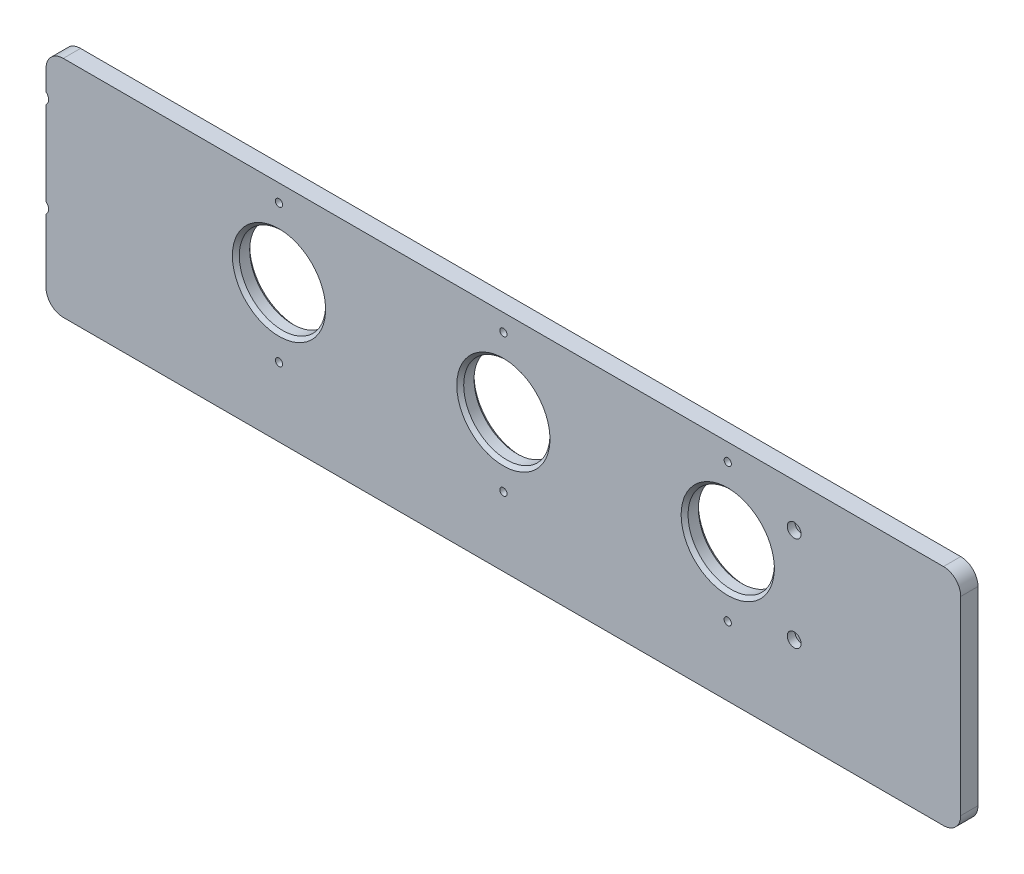
from build123d import *

# Parameters (mm, degrees)
SKETCH_1_W                   = 530
SKETCH_1_H                   = 130
EXTRUDE_1_DEPTH              = 10
HOLE_WIZARD_M4_1_D           = 4.5
HOLE_WIZARD_M4_1_CBORE_D     = 8
HOLE_WIZARD_M4_1_CBORE_DEPTH = 4.4
PATTERN_LINEAR_1_COUNT       = 2
PATTERN_LINEAR_1_PITCH       = 436
SKETCH_14_R                  = 25
CUT_EXTRUDE_1_DEPTH          = 274.03845883
CHAMFER_1_SIZE               = 2
HOLE_WIZARD_M5_2_D           = 4.2
FILLET_1_R                   = 10


with BuildPart() as part:
    # 草图1 → 凸台-拉伸1 (new body)
    with BuildSketch(Plane.XY):
        Rectangle(SKETCH_1_W, SKETCH_1_H)
    extrude(amount=EXTRUDE_1_DEPTH)

    # M4 六角凹头螺钉的柱形沉头孔1 (through all)
    with Locations(Plane(origin=(0, 0, 10), x_dir=(-1, 0, 0), z_dir=(0, 0, 1))):
        with Locations((-168.5, 15), (-168.5, -40)):
            hole_wizard_m4_1 = CounterBoreHole(HOLE_WIZARD_M4_1_D / 2, HOLE_WIZARD_M4_1_CBORE_D / 2, HOLE_WIZARD_M4_1_CBORE_DEPTH)

    # 阵列(线性)1: M4 六角凹头螺钉的柱形沉头孔1 ×2
    with Locations(*[(-i * PATTERN_LINEAR_1_PITCH, 0, 0) for i in range(1, PATTERN_LINEAR_1_COUNT)]):
        add(hole_wizard_m4_1, mode=Mode.SUBTRACT)

    # 草图14 → 切除-拉伸1 (cut, through all)
    with BuildSketch(Plane.XY.offset(10)):
        with Locations((-130, 15)):
            Circle(SKETCH_14_R)
        with Locations((0, 15)):
            Circle(SKETCH_14_R)
        with Locations((130, 15)):
            Circle(SKETCH_14_R)
    extrude(amount=-CUT_EXTRUDE_1_DEPTH, mode=Mode.SUBTRACT)

    # 倒角1
    chamfer_1_edges = [part.edges().sort_by_distance(p)[0] for p in [
        (-155, 15, 0),
        (-155, 15, 10),
        (-25, 15, 0),
        (-25, 15, 10),
        (105, 15, 0),
        (105, 15, 10),
    ]]
    chamfer(chamfer_1_edges, length=CHAMFER_1_SIZE)

    # M5 螺纹孔2 (through all)
    with Locations(Plane.XY.offset(10)):
        with Locations((130, 55), (-130, -25), (-130, 55), (0, 55), (0, -25), (130, -25)):
            Hole(HOLE_WIZARD_M5_2_D / 2)

    # 圆角1
    fillet_1_edges = [part.edges().sort_by_distance(p)[0] for p in [
        (265, -65, 5),
        (-265, -65, 5),
        (-265, 65, 5),
        (265, 65, 5),
    ]]
    fillet(fillet_1_edges, radius=FILLET_1_R)


solid = part.part
